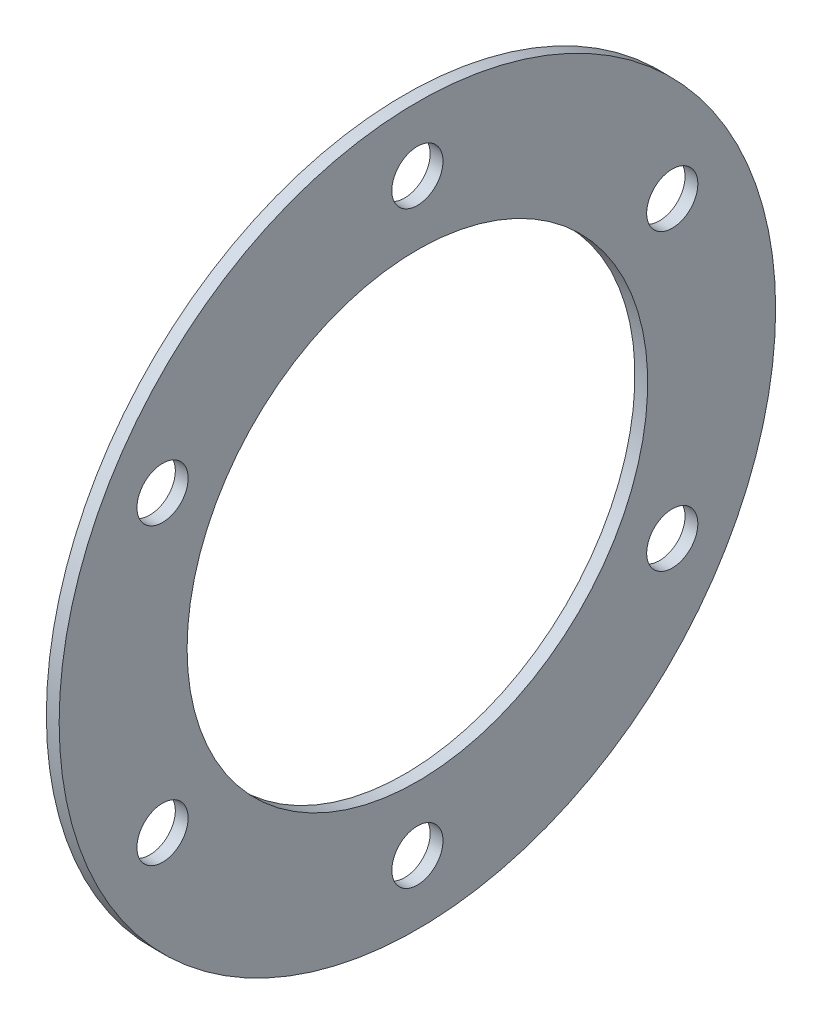
SolidWorks part; units mm, degrees
ref_plane "Front" through (0, 0, 0) normal (0, 0, 1) x (1, 0, 0)
ref_plane "Top" through (0, 0, 0) normal (0, 1, 0) x (1, 0, 0)
ref_plane "Right" through (0, 0, 0) normal (1, 0, 0) x (0, 0, -1)
sketch "Sketch1" plane through (0, 0, 0) normal (0, 0, 1) x (1, 0, 0)
  line L0 (0, 0) -> (38.117, 0) construction
  line L1 (0, 56) -> (2, 56)
  line L2 (0, 56) -> (0, 36)
  line L3 (0, 36) -> (2, 36)
  line L4 (2, 56) -> (2, 36)
  dimension "D1" = 2
  dimension "D2" = 20
  dimension "D3" = 36
revolve "Revolve1" add sketch "Sketch1" angle 360 about L0
sketch "Sketch2" plane through (2, 0, 0) normal (1, 0, 0) x (0, 0, -1)
  line L0 (0, 0) -> (0, 61.3864) construction
  line L1 (0, 0) -> (66.9211, 38.6369) construction
  line L2 (0, 0) -> (-60.8073, 35.1071) construction
  line L3 (0, 0) -> (0, -66.2857) construction
  line L4 (0, 0) -> (52.1705, 0) construction
  line L5 (0, 0) -> (39.8372, -23) construction
  line L6 (0, 0) -> (-39.8372, -23) construction
  circle A0 centre (0, 0) radius 46
  circle A1 centre (0, 46) radius 4
  circle A2 centre (39.8372, 23) radius 4
  circle A3 centre (-39.8372, 23) radius 4
  circle A4 centre (-39.8372, -23) radius 4
  circle A5 centre (0, -46) radius 4
  circle A6 centre (39.8372, -23) radius 4
  dimension "D1" = 92
  dimension "D2" = 8
  dimension "D3" = 60
  dimension "D4" = 8
  dimension "D5" = 60
  dimension "D6" = 60
extrude "Cut-Extrude1" cut sketch "Sketch2" against normal blind 10 contours A1 | A3 | A2 | A6 | A5 | A4
scale "Scale 1" bodies to scale 102 scale about centroid uniform scaling yes scale factor 1.875
